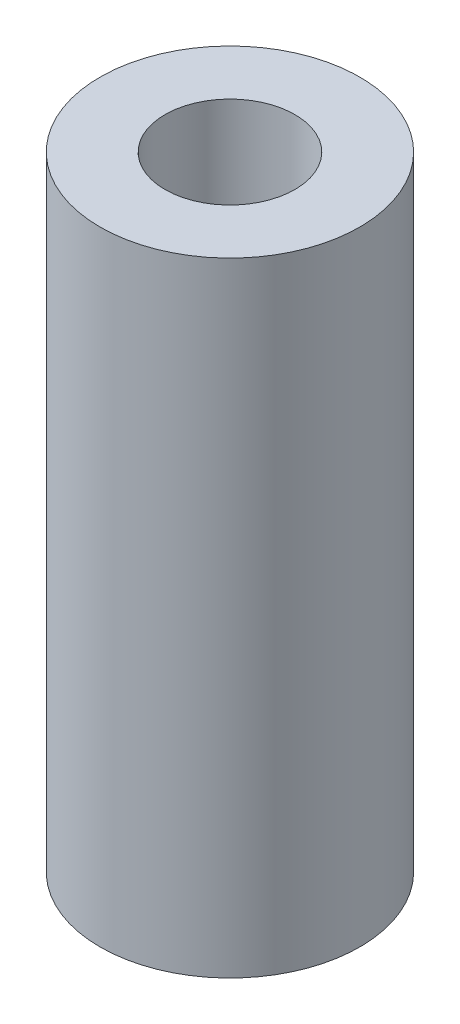
from build123d import *

# Parameters (mm, degrees)
SKETCH_1_R         = 2.5
EXTRUDE_1_DEPTH    = 12
HOLE_WIZARD_M3_1_D = 2.5


with BuildPart() as part:
    # 草图1 → 凸台-拉伸1 (new body)
    with BuildSketch(Plane(origin=(0, 0, 0), x_dir=(1, 0, 0), z_dir=(0, 1, 0))):
        with Locations(Location((0, 0, 0), (0, 0, 270))):
            Circle(SKETCH_1_R)
    extrude(amount=EXTRUDE_1_DEPTH)

    # M3 螺纹孔1 (through all)
    with Locations(Plane(origin=(0, 12, 0), x_dir=(1, 0, 0), z_dir=(0, 1, 0))):
        with Locations((0, 0)):
            Hole(HOLE_WIZARD_M3_1_D / 2)


solid = part.part
